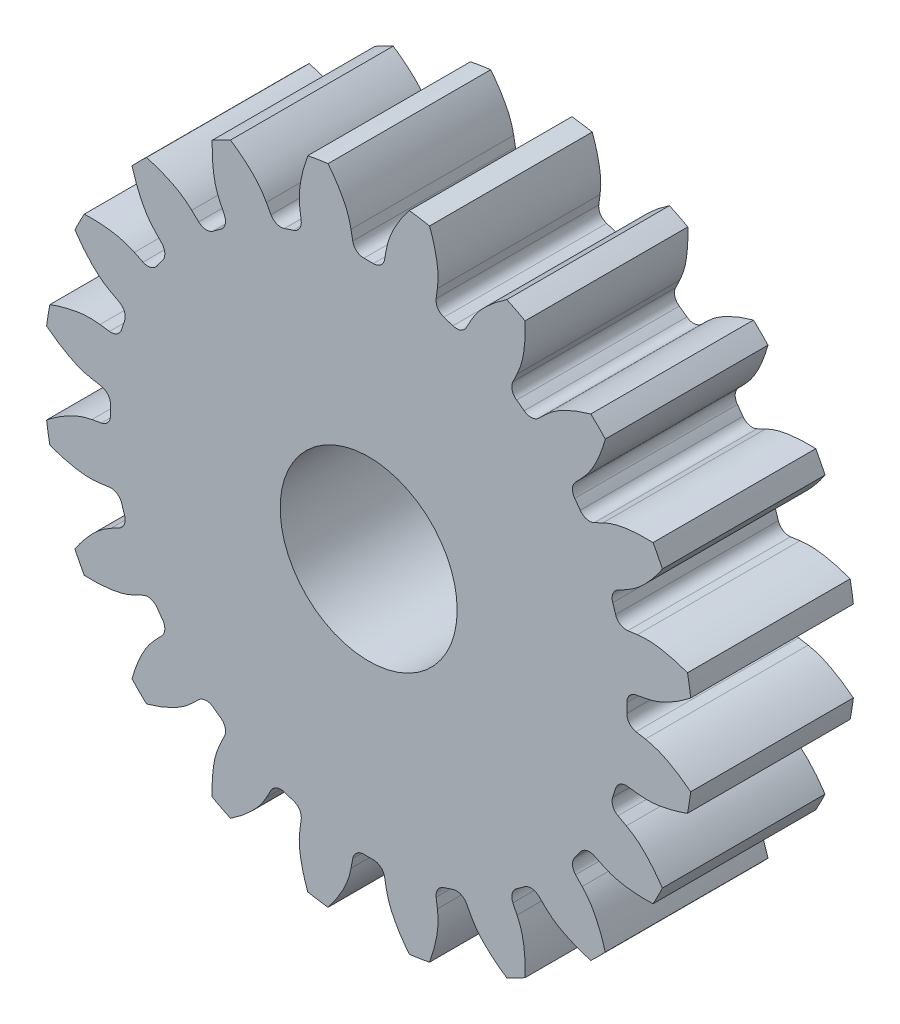
SolidWorks part; units mm, degrees
ref_plane "Front Plane" through (0, 0, 0) normal (0, 0, 1) x (1, 0, 0)
ref_plane "Top Plane" through (0, 0, 0) normal (0, 1, 0) x (1, 0, 0)
ref_plane "Right Plane" through (0, 0, 0) normal (1, 0, 0) x (0, 0, -1)
sketch "Model" plane through (0, 0, 0) normal (0, 0, 1) x (1, 0, 0)
  line L0 (-163.4597, -18.4626) -> (-162.9797, -18.3981)
  line L1 (-163.0447, -21.0831) -> (-162.5682, -20.9961)
  line L2 (-165.1645, -14.559) -> (-164.7278, -14.3493)
  line L3 (-163.96, -16.9231) -> (-163.5337, -16.6931)
  line L4 (-167.992, -11.3734) -> (-167.6416, -11.039)
  line L5 (-166.1159, -13.2495) -> (-165.7816, -12.899)
  line L6 (-171.6656, -9.2174) -> (-171.4357, -8.7911)
  line L7 (-169.3016, -10.4219) -> (-169.0919, -9.9853)
  line L8 (-175.8257, -8.3021) -> (-175.7387, -7.8256)
  line L9 (-173.2051, -8.7172) -> (-173.1406, -8.2371)
  line L10 (-180.0649, -8.7172) -> (-180.1295, -8.2371)
  line L11 (-177.4444, -8.3021) -> (-177.5314, -7.8256)
  line L12 (-183.9685, -10.4219) -> (-184.1782, -9.9853)
  line L13 (-181.6044, -9.2174) -> (-181.8344, -8.7911)
  line L14 (-187.1541, -13.2495) -> (-187.4885, -12.899)
  line L15 (-185.278, -11.3734) -> (-185.6285, -11.039)
  line L16 (-189.3101, -16.9231) -> (-189.7364, -16.6931)
  line L17 (-188.1056, -14.559) -> (-188.5422, -14.3493)
  line L18 (-190.2254, -21.0831) -> (-190.7019, -20.9961)
  line L19 (-189.8104, -18.4626) -> (-190.2904, -18.3981)
  line L20 (-189.8104, -25.3224) -> (-190.2904, -25.3869)
  line L21 (-190.2254, -22.7018) -> (-190.7019, -22.7888)
  line L22 (-188.1056, -29.2259) -> (-188.5422, -29.4356)
  line L23 (-189.3101, -26.8619) -> (-189.7364, -27.0919)
  line L24 (-185.278, -32.4116) -> (-185.6285, -32.7459)
  line L25 (-187.1541, -30.5355) -> (-187.4885, -30.8859)
  line L26 (-181.6044, -34.5676) -> (-181.8344, -34.9939)
  line L27 (-183.9685, -33.363) -> (-184.1782, -33.7997)
  line L28 (-177.4444, -35.4828) -> (-177.5314, -35.9593)
  line L29 (-180.0649, -35.0678) -> (-180.1295, -35.5478)
  line L30 (-173.2051, -35.0678) -> (-173.1406, -35.5478)
  line L31 (-175.8257, -35.4828) -> (-175.7387, -35.9593)
  line L32 (-169.3016, -33.363) -> (-169.0919, -33.7997)
  line L33 (-171.6656, -34.5676) -> (-171.4357, -34.9939)
  line L34 (-166.1159, -30.5355) -> (-165.7816, -30.8859)
  line L35 (-167.992, -32.4116) -> (-167.6416, -32.7459)
  line L36 (-163.96, -26.8619) -> (-163.5337, -27.0919)
  line L37 (-165.1645, -29.2259) -> (-164.7278, -29.4356)
  line L38 (-163.0447, -22.7018) -> (-162.5682, -22.7888)
  line L39 (-163.4597, -25.3224) -> (-162.9797, -25.3869)
  arc A0 (-164.0809, -18.0639) -> (-164.1524, -17.8366) centre (-176.635, -21.8925) ccw
  arc A1 (-163.51, -21.8925) -> (-163.5122, -21.6542) centre (-176.635, -21.8925) ccw
  arc A2 (-160.3382, -19.3113) -> (-160.4278, -18.7979) centre (-176.635, -21.8925) ccw
  arc A3 (-160.2648, -19.8272) -> (-160.3382, -19.3113) centre (-176.635, -21.8925) ccw
  arc A4 (-164.0809, -18.0639) -> (-163.4597, -18.4626) centre (-163.5357, -17.8977) ccw
  arc A5 (-163.0447, -21.0831) -> (-163.5122, -21.6542) centre (-162.9423, -21.6438) ccw
  arc A6 (-165.8784, -14.3718) -> (-166.0167, -14.1778) centre (-176.635, -21.8925) ccw
  arc A7 (-164.1524, -17.8366) -> (-164.2281, -17.6107) centre (-176.635, -21.8925) ccw
  arc A8 (-161.9334, -14.4016) -> (-162.1773, -13.9411) centre (-176.635, -21.8925) ccw
  arc A9 (-161.7042, -14.8696) -> (-161.9334, -14.4016) centre (-176.635, -21.8925) ccw
  arc A10 (-165.8784, -14.3718) -> (-165.1645, -14.559) centre (-165.4112, -14.0452) ccw
  arc A11 (-163.96, -16.9231) -> (-164.2281, -17.6107) centre (-163.6893, -17.4247) ccw
  arc A12 (-168.7289, -11.4159) -> (-168.9204, -11.2741) centre (-176.635, -21.8925) ccw
  arc A13 (-166.0167, -14.1778) -> (-166.1585, -13.9863) centre (-176.635, -21.8925) ccw
  arc A14 (-164.9678, -10.2252) -> (-165.3421, -9.8626) centre (-176.635, -21.8925) ccw
  arc A15 (-164.6051, -10.5995) -> (-164.9678, -10.2252) centre (-176.635, -21.8925) ccw
  arc A16 (-168.7289, -11.4159) -> (-167.992, -11.3734) centre (-168.3855, -10.961) ccw
  arc A17 (-166.1159, -13.2495) -> (-166.1585, -13.9863) centre (-165.7035, -13.6429) ccw
  arc A18 (-172.3532, -9.4855) -> (-172.5792, -9.4098) centre (-176.635, -21.8925) ccw
  arc A19 (-168.9204, -11.2741) -> (-169.1144, -11.1358) centre (-176.635, -21.8925) ccw
  arc A20 (-169.1442, -7.1909) -> (-169.6122, -6.9616) centre (-176.635, -21.8925) ccw
  arc A21 (-168.6837, -7.4348) -> (-169.1442, -7.1909) centre (-176.635, -21.8925) ccw
  arc A22 (-172.3532, -9.4855) -> (-171.6656, -9.2174) centre (-172.1673, -8.9467) ccw
  arc A23 (-169.3016, -10.4219) -> (-169.1144, -11.1358) centre (-168.7878, -10.6687) ccw
  arc A24 (-176.3968, -8.7696) -> (-176.635, -8.7675) centre (-176.635, -21.8925) ccw
  arc A25 (-172.5792, -9.4098) -> (-172.8065, -9.3383) centre (-176.635, -21.8925) ccw
  arc A26 (-174.0539, -5.5956) -> (-174.5698, -5.5222) centre (-176.635, -21.8925) ccw
  arc A27 (-173.5405, -5.6853) -> (-174.0539, -5.5956) centre (-176.635, -21.8925) ccw
  arc A28 (-176.3968, -8.7696) -> (-175.8257, -8.3021) centre (-176.3864, -8.1997) ccw
  arc A29 (-173.2051, -8.7172) -> (-172.8065, -9.3383) centre (-172.6402, -8.7931) ccw
  arc A30 (-180.4636, -9.3383) -> (-180.6909, -9.4098) centre (-176.635, -21.8925) ccw
  arc A31 (-176.635, -8.7675) -> (-176.8733, -8.7696) centre (-176.635, -21.8925) ccw
  arc A32 (-179.2162, -5.5956) -> (-179.7296, -5.6853) centre (-176.635, -21.8925) ccw
  arc A33 (-178.7003, -5.5222) -> (-179.2162, -5.5956) centre (-176.635, -21.8925) ccw
  arc A34 (-180.4636, -9.3383) -> (-180.0649, -8.7172) centre (-180.6299, -8.7931) ccw
  arc A35 (-177.4444, -8.3021) -> (-176.8733, -8.7696) centre (-176.8837, -8.1997) ccw
  arc A36 (-184.1557, -11.1358) -> (-184.3497, -11.2741) centre (-176.635, -21.8925) ccw
  arc A37 (-180.6909, -9.4098) -> (-180.9168, -9.4855) centre (-176.635, -21.8925) ccw
  arc A38 (-184.1259, -7.1909) -> (-184.5864, -7.4348) centre (-176.635, -21.8925) ccw
  arc A39 (-183.6579, -6.9616) -> (-184.1259, -7.1909) centre (-176.635, -21.8925) ccw
  arc A40 (-184.1557, -11.1358) -> (-183.9685, -10.4219) centre (-184.4823, -10.6687) ccw
  arc A41 (-181.6044, -9.2174) -> (-180.9168, -9.4855) centre (-181.1028, -8.9467) ccw
  arc A42 (-187.1116, -13.9863) -> (-187.2534, -14.1778) centre (-176.635, -21.8925) ccw
  arc A43 (-184.3497, -11.2741) -> (-184.5412, -11.4159) centre (-176.635, -21.8925) ccw
  arc A44 (-188.3023, -10.2252) -> (-188.6649, -10.5995) centre (-176.635, -21.8925) ccw
  arc A45 (-187.928, -9.8626) -> (-188.3023, -10.2252) centre (-176.635, -21.8925) ccw
  arc A46 (-187.1116, -13.9863) -> (-187.1541, -13.2495) centre (-187.5665, -13.6429) ccw
  arc A47 (-185.278, -11.3734) -> (-184.5412, -11.4159) centre (-184.8846, -10.961) ccw
  arc A48 (-189.042, -17.6107) -> (-189.1177, -17.8366) centre (-176.635, -21.8925) ccw
  arc A49 (-187.2534, -14.1778) -> (-187.3917, -14.3718) centre (-176.635, -21.8925) ccw
  arc A50 (-191.3367, -14.4016) -> (-191.5659, -14.8696) centre (-176.635, -21.8925) ccw
  arc A51 (-191.0928, -13.9411) -> (-191.3367, -14.4016) centre (-176.635, -21.8925) ccw
  arc A52 (-189.042, -17.6107) -> (-189.3101, -16.9231) centre (-189.5808, -17.4247) ccw
  arc A53 (-188.1056, -14.559) -> (-187.3917, -14.3718) centre (-187.8588, -14.0452) ccw
  arc A54 (-189.7579, -21.6542) -> (-189.76, -21.8925) centre (-176.635, -21.8925) ccw
  arc A55 (-189.1177, -17.8366) -> (-189.1892, -18.0639) centre (-176.635, -21.8925) ccw
  arc A56 (-192.9319, -19.3113) -> (-193.0053, -19.8272) centre (-176.635, -21.8925) ccw
  arc A57 (-192.8423, -18.7979) -> (-192.9319, -19.3113) centre (-176.635, -21.8925) ccw
  arc A58 (-189.7579, -21.6542) -> (-190.2254, -21.0831) centre (-190.3278, -21.6438) ccw
  arc A59 (-189.8104, -18.4626) -> (-189.1892, -18.0639) centre (-189.7344, -17.8977) ccw
  arc A60 (-189.1892, -25.721) -> (-189.1177, -25.9483) centre (-176.635, -21.8925) ccw
  arc A61 (-189.76, -21.8925) -> (-189.7579, -22.1308) centre (-176.635, -21.8925) ccw
  arc A62 (-192.9319, -24.4736) -> (-192.8423, -24.987) centre (-176.635, -21.8925) ccw
  arc A63 (-193.0053, -23.9577) -> (-192.9319, -24.4736) centre (-176.635, -21.8925) ccw
  arc A64 (-189.1892, -25.721) -> (-189.8104, -25.3224) centre (-189.7344, -25.8873) ccw
  arc A65 (-190.2254, -22.7018) -> (-189.7579, -22.1308) centre (-190.3278, -22.1411) ccw
  arc A66 (-187.3917, -29.4131) -> (-187.2534, -29.6071) centre (-176.635, -21.8925) ccw
  arc A67 (-189.1177, -25.9483) -> (-189.042, -26.1743) centre (-176.635, -21.8925) ccw
  arc A68 (-191.3367, -29.3833) -> (-191.0928, -29.8439) centre (-176.635, -21.8925) ccw
  arc A69 (-191.5659, -28.9153) -> (-191.3367, -29.3833) centre (-176.635, -21.8925) ccw
  arc A70 (-187.3917, -29.4131) -> (-188.1056, -29.2259) centre (-187.8588, -29.7397) ccw
  arc A71 (-189.3101, -26.8619) -> (-189.042, -26.1743) centre (-189.5808, -26.3602) ccw
  arc A72 (-184.5412, -32.369) -> (-184.3497, -32.5108) centre (-176.635, -21.8925) ccw
  arc A73 (-187.2534, -29.6071) -> (-187.1116, -29.7987) centre (-176.635, -21.8925) ccw
  arc A74 (-188.3023, -33.5597) -> (-187.928, -33.9224) centre (-176.635, -21.8925) ccw
  arc A75 (-188.6649, -33.1855) -> (-188.3023, -33.5597) centre (-176.635, -21.8925) ccw
  arc A76 (-184.5412, -32.369) -> (-185.278, -32.4116) centre (-184.8846, -32.824) ccw
  arc A77 (-187.1541, -30.5355) -> (-187.1116, -29.7987) centre (-187.5665, -30.142) ccw
  arc A78 (-180.9168, -34.2994) -> (-180.6909, -34.3751) centre (-176.635, -21.8925) ccw
  arc A79 (-184.3497, -32.5108) -> (-184.1557, -32.6491) centre (-176.635, -21.8925) ccw
  arc A80 (-184.1259, -36.5941) -> (-183.6579, -36.8233) centre (-176.635, -21.8925) ccw
  arc A81 (-184.5864, -36.3502) -> (-184.1259, -36.5941) centre (-176.635, -21.8925) ccw
  arc A82 (-180.9168, -34.2994) -> (-181.6044, -34.5676) centre (-181.1028, -34.8382) ccw
  arc A83 (-183.9685, -33.363) -> (-184.1557, -32.6491) centre (-184.4823, -33.1163) ccw
  arc A84 (-176.8733, -35.0153) -> (-176.635, -35.0175) centre (-176.635, -21.8925) ccw
  arc A85 (-180.6909, -34.3751) -> (-180.4636, -34.4467) centre (-176.635, -21.8925) ccw
  arc A86 (-179.2162, -38.1893) -> (-178.7003, -38.2627) centre (-176.635, -21.8925) ccw
  arc A87 (-179.7296, -38.0997) -> (-179.2162, -38.1893) centre (-176.635, -21.8925) ccw
  arc A88 (-176.8733, -35.0153) -> (-177.4444, -35.4828) centre (-176.8837, -35.5852) ccw
  arc A89 (-180.0649, -35.0678) -> (-180.4636, -34.4467) centre (-180.6299, -34.9919) ccw
  arc A90 (-172.8065, -34.4467) -> (-172.5792, -34.3751) centre (-176.635, -21.8925) ccw
  arc A91 (-176.635, -35.0175) -> (-176.3968, -35.0153) centre (-176.635, -21.8925) ccw
  arc A92 (-174.0539, -38.1893) -> (-173.5405, -38.0997) centre (-176.635, -21.8925) ccw
  arc A93 (-174.5698, -38.2627) -> (-174.0539, -38.1893) centre (-176.635, -21.8925) ccw
  arc A94 (-172.8065, -34.4467) -> (-173.2051, -35.0678) centre (-172.6402, -34.9919) ccw
  arc A95 (-175.8257, -35.4828) -> (-176.3968, -35.0153) centre (-176.3864, -35.5852) ccw
  arc A96 (-169.1144, -32.6491) -> (-168.9204, -32.5108) centre (-176.635, -21.8925) ccw
  arc A97 (-172.5792, -34.3751) -> (-172.3532, -34.2994) centre (-176.635, -21.8925) ccw
  arc A98 (-169.1442, -36.5941) -> (-168.6837, -36.3502) centre (-176.635, -21.8925) ccw
  arc A99 (-169.6122, -36.8233) -> (-169.1442, -36.5941) centre (-176.635, -21.8925) ccw
  arc A100 (-169.1144, -32.6491) -> (-169.3016, -33.363) centre (-168.7878, -33.1163) ccw
  arc A101 (-171.6656, -34.5676) -> (-172.3532, -34.2994) centre (-172.1673, -34.8382) ccw
  arc A102 (-166.1585, -29.7987) -> (-166.0167, -29.6071) centre (-176.635, -21.8925) ccw
  arc A103 (-168.9204, -32.5108) -> (-168.7289, -32.369) centre (-176.635, -21.8925) ccw
  arc A104 (-164.9678, -33.5597) -> (-164.6051, -33.1855) centre (-176.635, -21.8925) ccw
  arc A105 (-165.3421, -33.9224) -> (-164.9678, -33.5597) centre (-176.635, -21.8925) ccw
  arc A106 (-166.1585, -29.7987) -> (-166.1159, -30.5355) centre (-165.7035, -30.142) ccw
  arc A107 (-167.992, -32.4116) -> (-168.7289, -32.369) centre (-168.3855, -32.824) ccw
  arc A108 (-164.2281, -26.1743) -> (-164.1524, -25.9483) centre (-176.635, -21.8925) ccw
  arc A109 (-166.0167, -29.6071) -> (-165.8784, -29.4131) centre (-176.635, -21.8925) ccw
  arc A110 (-161.9334, -29.3833) -> (-161.7042, -28.9153) centre (-176.635, -21.8925) ccw
  arc A111 (-162.1773, -29.8439) -> (-161.9334, -29.3833) centre (-176.635, -21.8925) ccw
  arc A112 (-164.2281, -26.1743) -> (-163.96, -26.8619) centre (-163.6893, -26.3602) ccw
  arc A113 (-165.1645, -29.2259) -> (-165.8784, -29.4131) centre (-165.4112, -29.7397) ccw
  arc A114 (-163.5122, -22.1308) -> (-163.51, -21.8925) centre (-176.635, -21.8925) ccw
  arc A115 (-164.1524, -25.9483) -> (-164.0809, -25.721) centre (-176.635, -21.8925) ccw
  arc A116 (-160.3382, -24.4736) -> (-160.2648, -23.9577) centre (-176.635, -21.8925) ccw
  arc A117 (-160.4278, -24.987) -> (-160.3382, -24.4736) centre (-176.635, -21.8925) ccw
  arc A118 (-163.5122, -22.1308) -> (-163.0447, -22.7018) centre (-162.9423, -22.1411) ccw
  arc A119 (-163.4597, -25.3224) -> (-164.0809, -25.721) centre (-163.5357, -25.8873) ccw
  circle A120 centre (-176.635, -21.8925) radius 4.5
  spline S0 degree 3 poles (-162.9797, -18.3981) (-162.7773, -18.3709) (-162.3582, -18.3459) (-161.7222, -18.4275) (-161.0735, -18.5758) (-160.6431, -18.7162) (-160.4278, -18.7979) knots 0 0 0 0 0.613978 1.254721 1.921311 2.613663 2.613663 2.613663 2.613663 weights 1 1 1 1 1 1 1
  spline S1 degree 3 poles (-162.5682, -20.9961) (-162.3673, -20.9594) (-161.961, -20.8537) (-161.3814, -20.5795) (-160.8102, -20.238) (-160.4443, -19.9715) (-160.2648, -19.8272) knots 0 0 0 0 0.613978 1.254721 1.921311 2.613663 2.613663 2.613663 2.613663 weights 1 1 1 1 1 1 1
  spline S2 degree 3 poles (-164.7278, -14.3493) (-164.5438, -14.261) (-164.1529, -14.1077) (-163.5228, -13.9888) (-162.86, -13.9294) (-162.4073, -13.9299) (-162.1773, -13.9411) knots 0 0 0 0 0.613978 1.254721 1.921311 2.613663 2.613663 2.613663 2.613663 weights 1 1 1 1 1 1 1
  spline S3 degree 3 poles (-163.5337, -16.6931) (-163.354, -16.5961) (-163.0002, -16.37) (-162.5337, -15.9301) (-162.096, -15.4288) (-161.8303, -15.0623) (-161.7042, -14.8696) knots 0 0 0 0 0.613978 1.254721 1.921311 2.613663 2.613663 2.613663 2.613663 weights 1 1 1 1 1 1 1
  spline S4 degree 3 poles (-167.6416, -11.039) (-167.4939, -10.8981) (-167.1695, -10.6315) (-166.607, -10.3238) (-165.9949, -10.0624) (-165.5642, -9.923) (-165.3421, -9.8626) knots 0 0 0 0 0.613978 1.254721 1.921311 2.613663 2.613663 2.613663 2.613663 weights 1 1 1 1 1 1 1
  spline S5 degree 3 poles (-165.7816, -12.899) (-165.6407, -12.7513) (-165.3741, -12.4269) (-165.0663, -11.8644) (-164.805, -11.2524) (-164.6656, -10.8216) (-164.6051, -10.5995) knots 0 0 0 0 0.613978 1.254721 1.921311 2.613663 2.613663 2.613663 2.613663 weights 1 1 1 1 1 1 1
  spline S6 degree 3 poles (-171.4357, -8.7911) (-171.3387, -8.6114) (-171.1126, -8.2577) (-170.6727, -7.7911) (-170.1714, -7.3534) (-169.8048, -7.0877) (-169.6122, -6.9616) knots 0 0 0 0 0.613978 1.254721 1.921311 2.613663 2.613663 2.613663 2.613663 weights 1 1 1 1 1 1 1
  spline S7 degree 3 poles (-169.0919, -9.9853) (-169.0035, -9.8012) (-168.8503, -9.4104) (-168.7314, -8.7803) (-168.672, -8.1174) (-168.6725, -7.6647) (-168.6837, -7.4348) knots 0 0 0 0 0.613978 1.254721 1.921311 2.613663 2.613663 2.613663 2.613663 weights 1 1 1 1 1 1 1
  spline S8 degree 3 poles (-175.7387, -7.8256) (-175.702, -7.6248) (-175.5963, -7.2185) (-175.3221, -6.6388) (-174.9806, -6.0676) (-174.714, -5.7017) (-174.5698, -5.5222) knots 0 0 0 0 0.613978 1.254721 1.921311 2.613663 2.613663 2.613663 2.613663 weights 1 1 1 1 1 1 1
  spline S9 degree 3 poles (-173.1406, -8.2371) (-173.1134, -8.0348) (-173.0885, -7.6157) (-173.1701, -6.9797) (-173.3184, -6.3309) (-173.4588, -5.9005) (-173.5405, -5.6853) knots 0 0 0 0 0.613978 1.254721 1.921311 2.613663 2.613663 2.613663 2.613663 weights 1 1 1 1 1 1 1
  spline S10 degree 3 poles (-180.1295, -8.2371) (-180.1566, -8.0348) (-180.1816, -7.6157) (-180.1, -6.9797) (-179.9517, -6.3309) (-179.8113, -5.9005) (-179.7296, -5.6853) knots 0 0 0 0 0.613978 1.254721 1.921311 2.613663 2.613663 2.613663 2.613663 weights 1 1 1 1 1 1 1
  spline S11 degree 3 poles (-177.5314, -7.8256) (-177.5681, -7.6248) (-177.6738, -7.2185) (-177.948, -6.6388) (-178.2895, -6.0676) (-178.5561, -5.7017) (-178.7003, -5.5222) knots 0 0 0 0 0.613978 1.254721 1.921311 2.613663 2.613663 2.613663 2.613663 weights 1 1 1 1 1 1 1
  spline S12 degree 3 poles (-184.1782, -9.9853) (-184.2666, -9.8012) (-184.4198, -9.4104) (-184.5387, -8.7803) (-184.5981, -8.1174) (-184.5976, -7.6647) (-184.5864, -7.4348) knots 0 0 0 0 0.613978 1.254721 1.921311 2.613663 2.613663 2.613663 2.613663 weights 1 1 1 1 1 1 1
  spline S13 degree 3 poles (-181.8344, -8.7911) (-181.9314, -8.6114) (-182.1575, -8.2577) (-182.5974, -7.7911) (-183.0987, -7.3534) (-183.4653, -7.0877) (-183.6579, -6.9616) knots 0 0 0 0 0.613978 1.254721 1.921311 2.613663 2.613663 2.613663 2.613663 weights 1 1 1 1 1 1 1
  spline S14 degree 3 poles (-187.4885, -12.899) (-187.6294, -12.7513) (-187.896, -12.4269) (-188.2038, -11.8644) (-188.4651, -11.2524) (-188.6045, -10.8216) (-188.6649, -10.5995) knots 0 0 0 0 0.613978 1.254721 1.921311 2.613663 2.613663 2.613663 2.613663 weights 1 1 1 1 1 1 1
  spline S15 degree 3 poles (-185.6285, -11.039) (-185.7762, -10.8981) (-186.1006, -10.6315) (-186.6631, -10.3238) (-187.2751, -10.0624) (-187.7059, -9.923) (-187.928, -9.8626) knots 0 0 0 0 0.613978 1.254721 1.921311 2.613663 2.613663 2.613663 2.613663 weights 1 1 1 1 1 1 1
  spline S16 degree 3 poles (-189.7364, -16.6931) (-189.9161, -16.5961) (-190.2699, -16.37) (-190.7364, -15.9301) (-191.1741, -15.4288) (-191.4398, -15.0623) (-191.5659, -14.8696) knots 0 0 0 0 0.613978 1.254721 1.921311 2.613663 2.613663 2.613663 2.613663 weights 1 1 1 1 1 1 1
  spline S17 degree 3 poles (-188.5422, -14.3493) (-188.7263, -14.261) (-189.1171, -14.1077) (-189.7472, -13.9888) (-190.4101, -13.9294) (-190.8628, -13.9299) (-191.0928, -13.9411) knots 0 0 0 0 0.613978 1.254721 1.921311 2.613663 2.613663 2.613663 2.613663 weights 1 1 1 1 1 1 1
  spline S18 degree 3 poles (-190.7019, -20.9961) (-190.9027, -20.9594) (-191.3091, -20.8537) (-191.8887, -20.5795) (-192.4599, -20.238) (-192.8258, -19.9715) (-193.0053, -19.8272) knots 0 0 0 0 0.613978 1.254721 1.921311 2.613663 2.613663 2.613663 2.613663 weights 1 1 1 1 1 1 1
  spline S19 degree 3 poles (-190.2904, -18.3981) (-190.4928, -18.3709) (-190.9119, -18.3459) (-191.5479, -18.4275) (-192.1966, -18.5758) (-192.627, -18.7162) (-192.8423, -18.7979) knots 0 0 0 0 0.613978 1.254721 1.921311 2.613663 2.613663 2.613663 2.613663 weights 1 1 1 1 1 1 1
  spline S20 degree 3 poles (-190.2904, -25.3869) (-190.4928, -25.4141) (-190.9119, -25.439) (-191.5479, -25.3574) (-192.1966, -25.2091) (-192.627, -25.0687) (-192.8423, -24.987) knots 0 0 0 0 0.613978 1.254721 1.921311 2.613663 2.613663 2.613663 2.613663 weights 1 1 1 1 1 1 1
  spline S21 degree 3 poles (-190.7019, -22.7888) (-190.9027, -22.8255) (-191.3091, -22.9312) (-191.8887, -23.2054) (-192.4599, -23.547) (-192.8258, -23.8135) (-193.0053, -23.9577) knots 0 0 0 0 0.613978 1.254721 1.921311 2.613663 2.613663 2.613663 2.613663 weights 1 1 1 1 1 1 1
  spline S22 degree 3 poles (-188.5422, -29.4356) (-188.7263, -29.524) (-189.1171, -29.6772) (-189.7472, -29.7961) (-190.4101, -29.8556) (-190.8628, -29.855) (-191.0928, -29.8439) knots 0 0 0 0 0.613978 1.254721 1.921311 2.613663 2.613663 2.613663 2.613663 weights 1 1 1 1 1 1 1
  spline S23 degree 3 poles (-189.7364, -27.0919) (-189.9161, -27.1888) (-190.2699, -27.4149) (-190.7364, -27.8548) (-191.1741, -28.3561) (-191.4398, -28.7227) (-191.5659, -28.9153) knots 0 0 0 0 0.613978 1.254721 1.921311 2.613663 2.613663 2.613663 2.613663 weights 1 1 1 1 1 1 1
  spline S24 degree 3 poles (-185.6285, -32.7459) (-185.7762, -32.8869) (-186.1006, -33.1534) (-186.6631, -33.4612) (-187.2751, -33.7225) (-187.7059, -33.8619) (-187.928, -33.9224) knots 0 0 0 0 0.613978 1.254721 1.921311 2.613663 2.613663 2.613663 2.613663 weights 1 1 1 1 1 1 1
  spline S25 degree 3 poles (-187.4885, -30.8859) (-187.6294, -31.0336) (-187.896, -31.358) (-188.2038, -31.9206) (-188.4651, -32.5326) (-188.6045, -32.9633) (-188.6649, -33.1855) knots 0 0 0 0 0.613978 1.254721 1.921311 2.613663 2.613663 2.613663 2.613663 weights 1 1 1 1 1 1 1
  spline S26 degree 3 poles (-181.8344, -34.9939) (-181.9314, -35.1735) (-182.1575, -35.5273) (-182.5974, -35.9938) (-183.0987, -36.4315) (-183.4653, -36.6972) (-183.6579, -36.8233) knots 0 0 0 0 0.613978 1.254721 1.921311 2.613663 2.613663 2.613663 2.613663 weights 1 1 1 1 1 1 1
  spline S27 degree 3 poles (-184.1782, -33.7997) (-184.2666, -33.9837) (-184.4198, -34.3746) (-184.5387, -35.0047) (-184.5981, -35.6675) (-184.5976, -36.1202) (-184.5864, -36.3502) knots 0 0 0 0 0.613978 1.254721 1.921311 2.613663 2.613663 2.613663 2.613663 weights 1 1 1 1 1 1 1
  spline S28 degree 3 poles (-177.5314, -35.9593) (-177.5681, -36.1602) (-177.6738, -36.5665) (-177.948, -37.1461) (-178.2895, -37.7173) (-178.5561, -38.0833) (-178.7003, -38.2627) knots 0 0 0 0 0.613978 1.254721 1.921311 2.613663 2.613663 2.613663 2.613663 weights 1 1 1 1 1 1 1
  spline S29 degree 3 poles (-180.1295, -35.5478) (-180.1566, -35.7502) (-180.1816, -36.1693) (-180.1, -36.8053) (-179.9517, -37.454) (-179.8113, -37.8844) (-179.7296, -38.0997) knots 0 0 0 0 0.613978 1.254721 1.921311 2.613663 2.613663 2.613663 2.613663 weights 1 1 1 1 1 1 1
  spline S30 degree 3 poles (-173.1406, -35.5478) (-173.1134, -35.7502) (-173.0885, -36.1693) (-173.1701, -36.8053) (-173.3184, -37.454) (-173.4588, -37.8844) (-173.5405, -38.0997) knots 0 0 0 0 0.613978 1.254721 1.921311 2.613663 2.613663 2.613663 2.613663 weights 1 1 1 1 1 1 1
  spline S31 degree 3 poles (-175.7387, -35.9593) (-175.702, -36.1602) (-175.5963, -36.5665) (-175.3221, -37.1461) (-174.9806, -37.7173) (-174.714, -38.0833) (-174.5698, -38.2627) knots 0 0 0 0 0.613978 1.254721 1.921311 2.613663 2.613663 2.613663 2.613663 weights 1 1 1 1 1 1 1
  spline S32 degree 3 poles (-169.0919, -33.7997) (-169.0035, -33.9837) (-168.8503, -34.3746) (-168.7314, -35.0047) (-168.672, -35.6675) (-168.6725, -36.1202) (-168.6837, -36.3502) knots 0 0 0 0 0.613978 1.254721 1.921311 2.613663 2.613663 2.613663 2.613663 weights 1 1 1 1 1 1 1
  spline S33 degree 3 poles (-171.4357, -34.9939) (-171.3387, -35.1735) (-171.1126, -35.5273) (-170.6727, -35.9938) (-170.1714, -36.4315) (-169.8048, -36.6972) (-169.6122, -36.8233) knots 0 0 0 0 0.613978 1.254721 1.921311 2.613663 2.613663 2.613663 2.613663 weights 1 1 1 1 1 1 1
  spline S34 degree 3 poles (-165.7816, -30.8859) (-165.6407, -31.0336) (-165.3741, -31.358) (-165.0663, -31.9206) (-164.805, -32.5326) (-164.6656, -32.9633) (-164.6051, -33.1855) knots 0 0 0 0 0.613978 1.254721 1.921311 2.613663 2.613663 2.613663 2.613663 weights 1 1 1 1 1 1 1
  spline S35 degree 3 poles (-167.6416, -32.7459) (-167.4939, -32.8869) (-167.1695, -33.1534) (-166.607, -33.4612) (-165.9949, -33.7225) (-165.5642, -33.8619) (-165.3421, -33.9224) knots 0 0 0 0 0.613978 1.254721 1.921311 2.613663 2.613663 2.613663 2.613663 weights 1 1 1 1 1 1 1
  spline S36 degree 3 poles (-163.5337, -27.0919) (-163.354, -27.1888) (-163.0002, -27.4149) (-162.5337, -27.8548) (-162.096, -28.3561) (-161.8303, -28.7227) (-161.7042, -28.9153) knots 0 0 0 0 0.613978 1.254721 1.921311 2.613663 2.613663 2.613663 2.613663 weights 1 1 1 1 1 1 1
  spline S37 degree 3 poles (-164.7278, -29.4356) (-164.5438, -29.524) (-164.1529, -29.6772) (-163.5228, -29.7961) (-162.86, -29.8556) (-162.4073, -29.855) (-162.1773, -29.8439) knots 0 0 0 0 0.613978 1.254721 1.921311 2.613663 2.613663 2.613663 2.613663 weights 1 1 1 1 1 1 1
  spline S38 degree 3 poles (-162.5682, -22.7888) (-162.3673, -22.8255) (-161.961, -22.9312) (-161.3814, -23.2054) (-160.8102, -23.547) (-160.4443, -23.8135) (-160.2648, -23.9577) knots 0 0 0 0 0.613978 1.254721 1.921311 2.613663 2.613663 2.613663 2.613663 weights 1 1 1 1 1 1 1
  spline S39 degree 3 poles (-162.9797, -25.3869) (-162.7773, -25.4141) (-162.3582, -25.439) (-161.7222, -25.3574) (-161.0735, -25.2091) (-160.6431, -25.0687) (-160.4278, -24.987) knots 0 0 0 0 0.613978 1.254721 1.921311 2.613663 2.613663 2.613663 2.613663 weights 1 1 1 1 1 1 1
extrude "Boss-Extrude1" add sketch "Model" along normal blind 8.27
